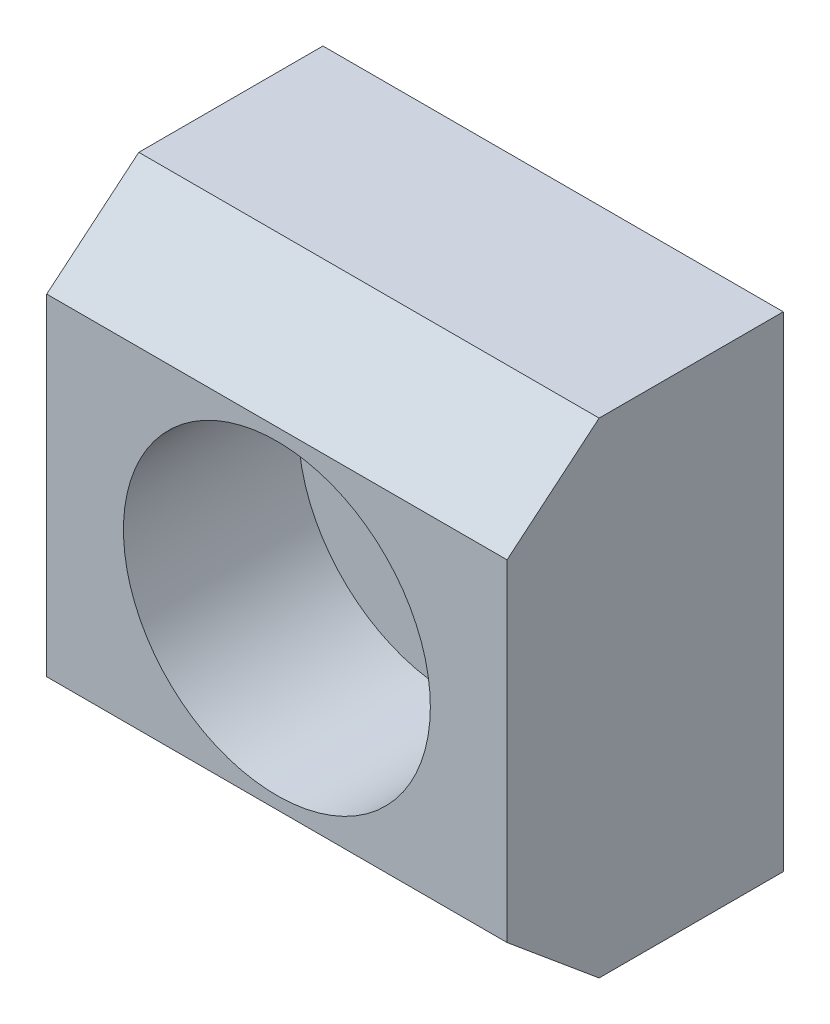
SolidWorks part; units mm, degrees
material "SUS304"
ref_plane "前视基准面" through (0, 0, 0) normal (0, 0, 1) x (1, 0, 0)
ref_plane "上视基准面" through (0, 0, 0) normal (0, 1, 0) x (1, 0, 0)
ref_plane "右视基准面" through (0, 0, 0) normal (1, 0, 0) x (0, 0, -1)
sketch "草图1" plane through (0, 0, 0) normal (0, 0, 1) x (1, 0, 0)
  line L1 (-7.5, 7.9) -> (7.5, 7.9)
  line L2 (-7.5, 7.9) -> (-7.5, -7.9)
  line L3 (-7.5, -7.9) -> (7.5, -7.9)
  line L4 (7.5, 7.9) -> (7.5, -7.9)
  line L5 (-7.5, 7.9) -> (7.5, -7.9) construction
  line L6 (-7.5, -7.9) -> (7.5, 7.9) construction
  point P0 (0, 0)
  dimension "D1" = 15.8
  dimension "D2" = 15
extrude "凸台-拉伸1" add sketch "草图1" along normal mid plane 9
hole_wizard "M4 沉头孔1" positions "草图3" profile "草图2" counterbore size "M5" standard "GB" end condition up to next
sketch "草图3" plane through (0, 0, 4.5) normal (0, 0, 1) x (1, 0, 0)
  point P1 (0, 0)
sketch "草图2" plane through (0, 0, 4.5) normal (1, 0, 0) x (0, -1, 0)
  line L0 (0, 0) -> (0, 9)
  line L1 (0, 9) -> (2.75, 9)
  line L3 (2.75, 9) -> (2.75, 5.7)
  line L4 (2.75, 5.7) -> (5, 5.7)
  line L5 (5, 5.7) -> (5, 0)
  line L7 (5, 0) -> (0, 0)
  line L11 (0, -6.35) -> (0, 107.95) construction
  dimension "通孔孔直径" = 5.5
  dimension "通孔孔深度" = 9
  dimension "柱形沉头孔直径" = 10
  dimension "柱形沉头孔深度" = 5.7
sketch "草图4" plane through (7.5, 0, 0) normal (1, 0, 0) x (0, 0, -1)
  line L0 (-4.5, -7.9) -> (-4.5, -5.4)
  line L1 (-4.5, -7.9) -> (-4.5, 7.9) construction
  line L2 (-4.5, -5.4) -> (-1.5, -7.9)
  line L3 (-4.5, -7.9) -> (4.5, -7.9) construction
  line L4 (-1.5, -7.9) -> (-4.5, -7.9)
  line L5 (-4.5, 5.4) -> (-4.5, 7.9)
  line L6 (-4.5, 7.9) -> (-1.5, 7.9)
  line L7 (-4.5, 7.9) -> (4.5, 7.9) construction
  line L8 (-1.5, 7.9) -> (-4.5, 5.4)
  dimension "D1" = 2.5
  dimension "D2" = 3
extrude "切除-拉伸1" cut sketch "草图4" against normal through all
